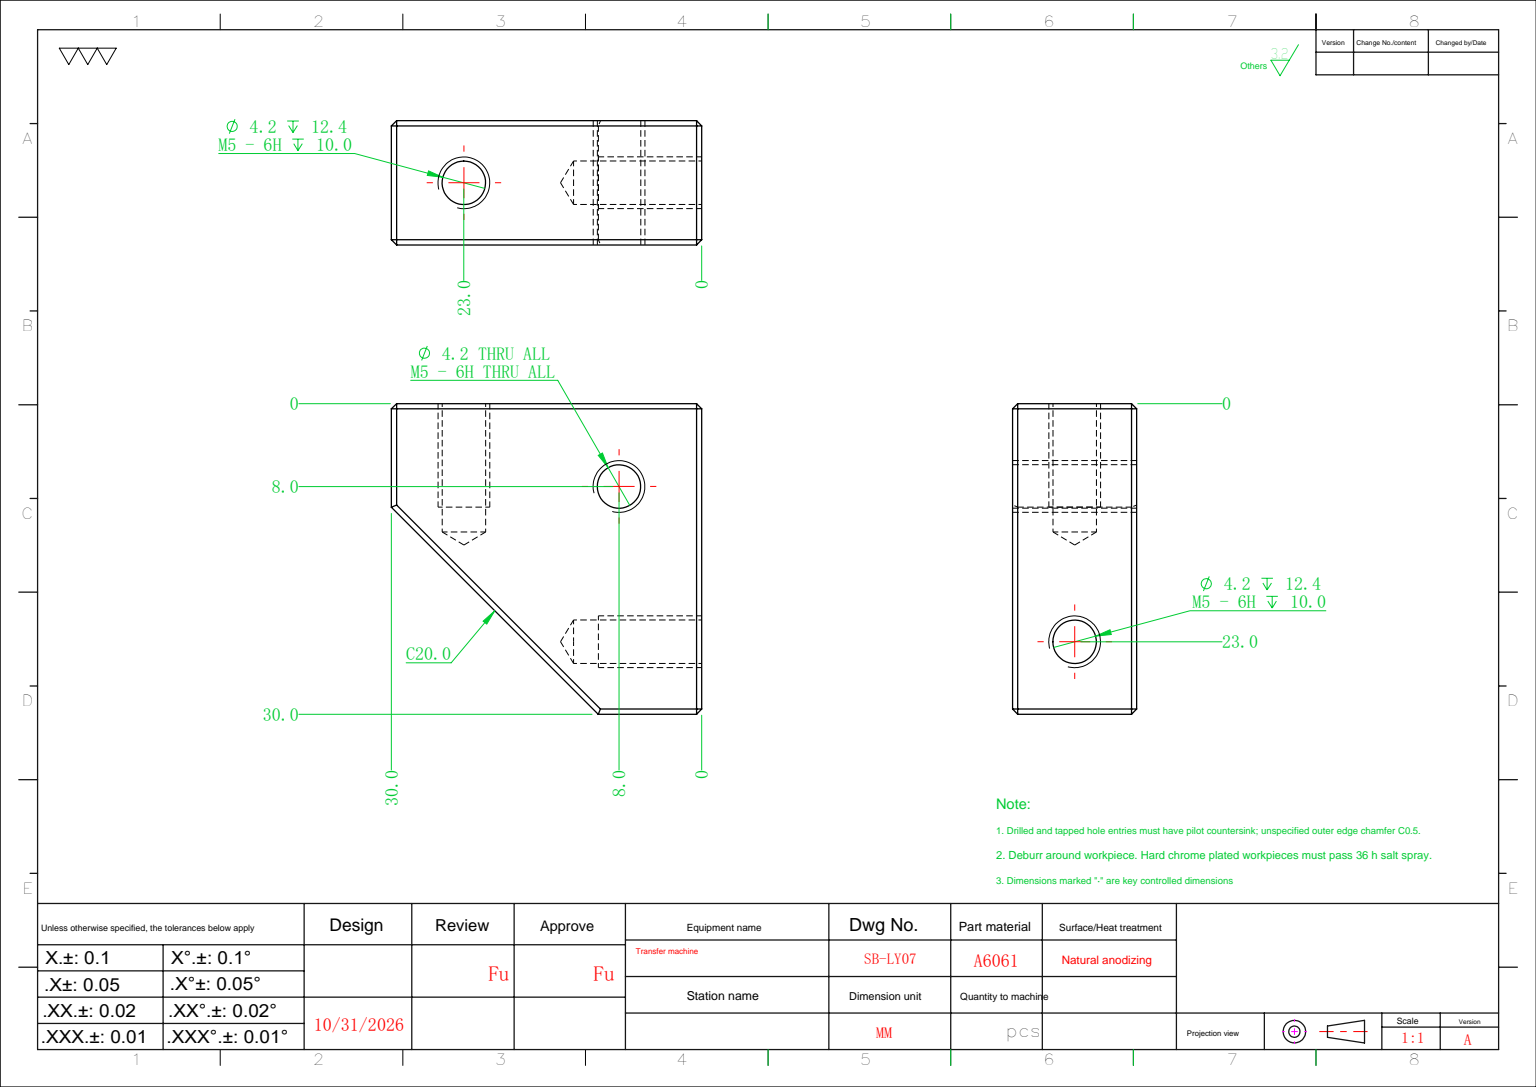
from build123d import *

# Parameters (mm, degrees)
SKETCH_1_W             = 30
SKETCH_1_H             = 30
EXTRUDE_1_DEPTH        = 12
CHAMFER_1_SIZE         = 20
HOLE_WIZARD_M5_1_D     = 4.2
HOLE_WIZARD_M5_2_D     = 4.2
HOLE_WIZARD_M5_2_DEPTH = 12.4
HOLE_WIZARD_M5_2_TIP   = 1.2618073
HOLE_WIZARD_M5_3_D     = 4.2
HOLE_WIZARD_M5_3_DEPTH = 12.4
HOLE_WIZARD_M5_3_TIP   = 1.2618073
CHAMFER_2_SIZE         = 0.5


with BuildPart() as part:
    # 草图1 → 凸台-拉伸1 (new body)
    with BuildSketch(Plane.XY):
        Rectangle(SKETCH_1_W, SKETCH_1_H)
    extrude(amount=EXTRUDE_1_DEPTH)

    # 倒角1
    chamfer_1_edges = [part.edges().sort_by_distance(p)[0] for p in [
        (15, 15, 6),
    ]]
    chamfer(chamfer_1_edges, length=CHAMFER_1_SIZE)

    # M5 螺纹孔1 (through all)
    with Locations(Plane.XY.offset(12)):
        with Locations((-7, -7)):
            Hole(HOLE_WIZARD_M5_1_D / 2)

    # M5 螺纹孔2
    with Locations(Plane(origin=(0, -15, 0), x_dir=(-1, 0, 0), z_dir=(0, -1, 0))):
        with Locations((-8, -6)):
            Hole(HOLE_WIZARD_M5_2_D / 2, depth=HOLE_WIZARD_M5_2_DEPTH)
            with Locations((0, 0, -(HOLE_WIZARD_M5_2_DEPTH + HOLE_WIZARD_M5_2_TIP / 2))):  # 118° drill point
                Cone(0, HOLE_WIZARD_M5_2_D / 2, HOLE_WIZARD_M5_2_TIP, mode=Mode.SUBTRACT)

    # M5 螺纹孔3
    with Locations(Plane.ZY.offset(15)):
        with Locations((6, 8)):
            Hole(HOLE_WIZARD_M5_3_D / 2, depth=HOLE_WIZARD_M5_3_DEPTH)
            with Locations((0, 0, -(HOLE_WIZARD_M5_3_DEPTH + HOLE_WIZARD_M5_3_TIP / 2))):  # 118° drill point
                Cone(0, HOLE_WIZARD_M5_3_D / 2, HOLE_WIZARD_M5_3_TIP, mode=Mode.SUBTRACT)

    # 倒角2
    chamfer_2_edges = [part.edges().sort_by_distance(p)[0] for p in [
        (-15, 0, 12),
        (-10, 15, 0),
        (-10, 15, 12),
        (5, 5, 0),
        (5, 5, 12),
        (0, -15, 12),
        (15, -10, 12),
        (0, -15, 0),
        (-15, 0, 0),
        (15, -10, 0),
        (15, -15, 6),
        (-15, -15, 6),
        (-15, 15, 6),
    ]]
    chamfer(chamfer_2_edges, length=CHAMFER_2_SIZE)


solid = part.part
